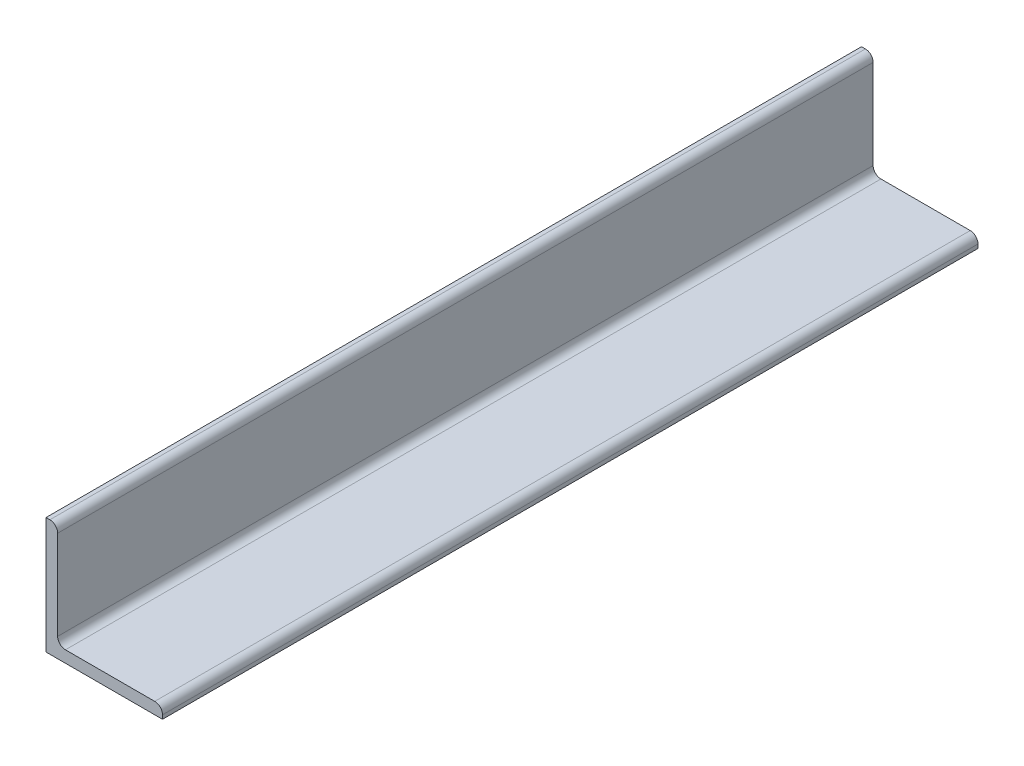
SolidWorks part; units mm, degrees
material "Plain Carbon Steel"
ref_plane "Front Plane" through (0, 0, 0) normal (0, 0, 1) x (1, 0, 0)
ref_plane "Top Plane" through (0, 0, 0) normal (0, 1, 0) x (1, 0, 0)
ref_plane "Right Plane" through (0, 0, 0) normal (1, 0, 0) x (0, 0, -1)
sketch "Sketch1" plane through (0, 0, 0) normal (0, 0, 1) x (1, 0, 0)
  line L0 (0, 0) -> (30, 0)
  line L1 (0, 0) -> (0, 30)
  line L2 (5, 3) -> (28, 3)
  line L3 (3, 5) -> (3, 28)
  line L4 (0, 30) -> (1, 30)
  line L5 (30, 1) -> (30, 0)
  line L6 (3, 3) -> (30, 3) construction
  line L7 (3, 3) -> (3, 30) construction
  arc A0 (30, 1) -> (28, 3) centre (28, 1) ccw
  arc A1 (5, 3) -> (3, 5) centre (5, 5) cw
  arc A2 (3, 28) -> (1, 30) centre (1, 28) ccw
  dimension "D4" = 2
  dimension "D1" = 30
  dimension "D2" = 30
  dimension "D3" = 3
extrude "Boss-Extrude1" add sketch "Sketch1" along normal blind 210
